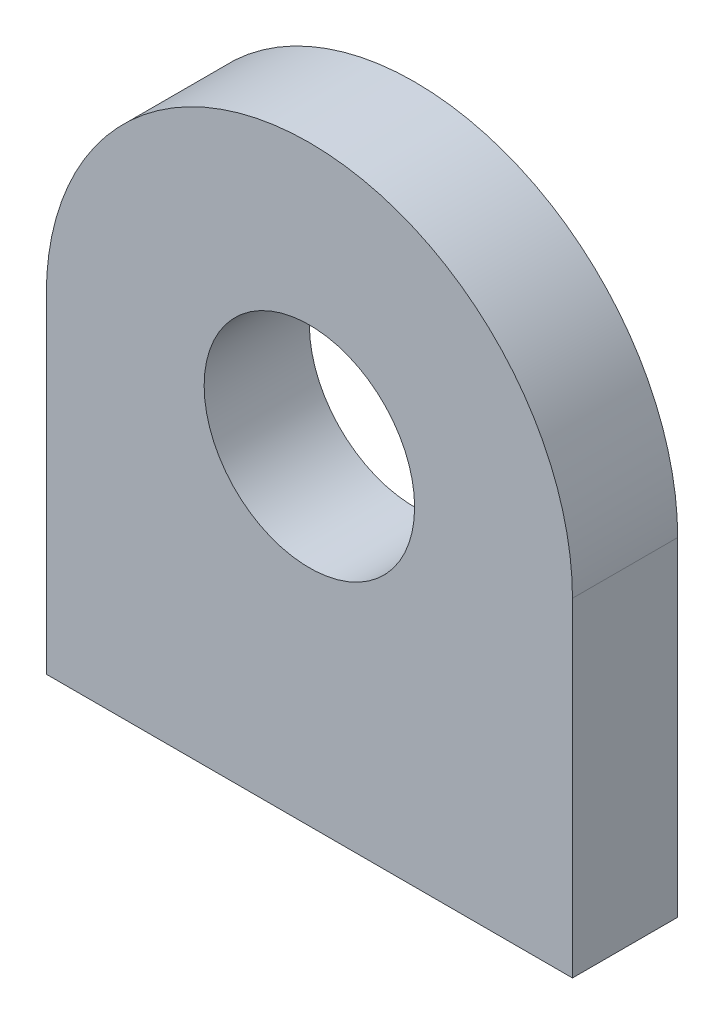
from build123d import *

# Parameters (mm, degrees)
SKETCH1_R           = 8
BOSS_EXTRUDE1_DEPTH = 8


with BuildPart() as part:
    # Sketch1 → Boss-Extrude1 (new body)
    with BuildSketch(Plane.XY):
        with BuildLine():
            Line((-20, 0), (-20, -25))
            Line((-20, -25), (20, -25))
            Line((20, -25), (20, 0))
            ThreePointArc((20, 0), (0, 20), (-20, 0))
        make_face()
        Circle(SKETCH1_R, mode=Mode.SUBTRACT)
    extrude(amount=BOSS_EXTRUDE1_DEPTH)


solid = part.part
